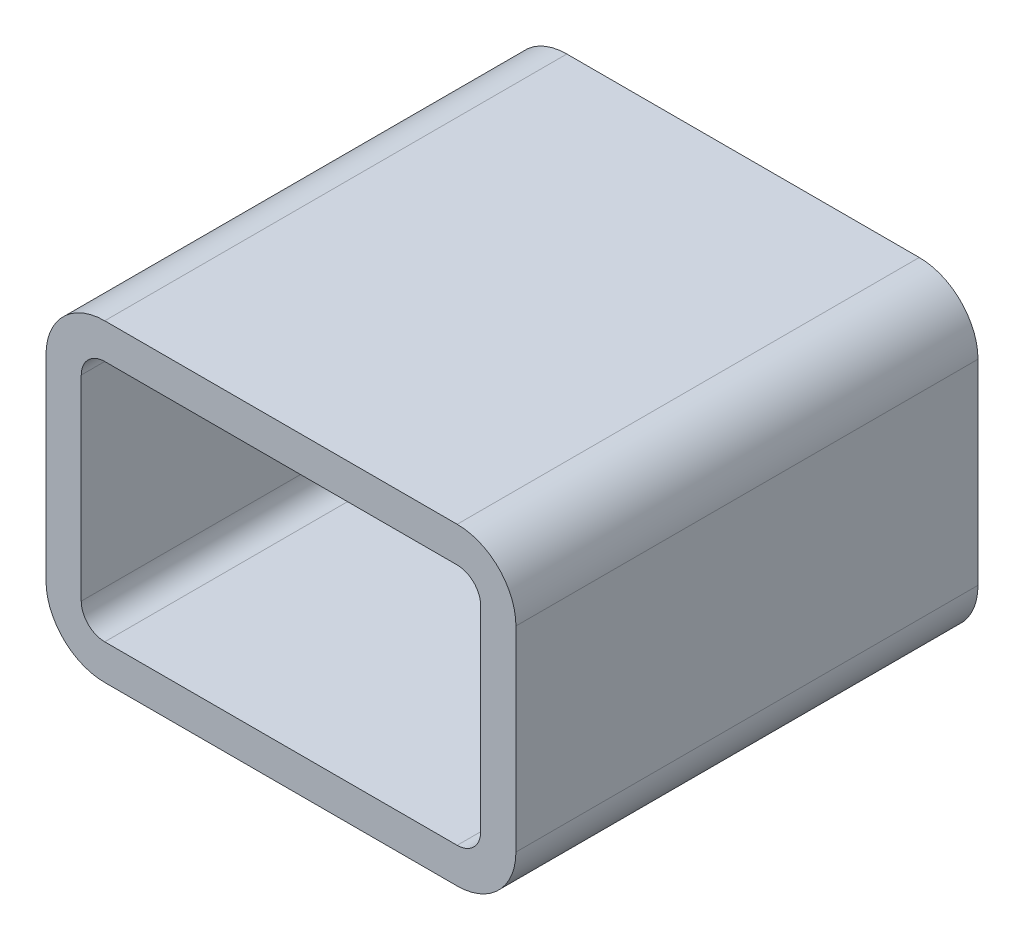
SolidWorks part; units mm, degrees
material "普通碳钢"
ref_plane "前视基准面" through (0, 0, 0) normal (0, 0, 1) x (1, 0, 0)
ref_plane "上视基准面" through (0, 0, 0) normal (0, 1, 0) x (1, 0, 0)
ref_plane "右视基准面" through (0, 0, 0) normal (1, 0, 0) x (0, 0, -1)
sketch "草图1" plane through (0, 0, 0) normal (0, 0, 1) x (1, 0, 0)
  line L0 (-101.745, 0) -> (99.7101, 0) construction
  line L1 (0, 68.9021) -> (0, -49.677) construction
  line L2 (-60, 40) -> (60, 40)
  line L3 (60, 40) -> (60, -40)
  line L4 (60, -40) -> (-60, -40)
  line L5 (-60, -40) -> (-60, 40)
  line L6 (-51, 31) -> (51, 31)
  line L7 (51, 31) -> (51, -31)
  line L8 (51, -31) -> (-51, -31)
  line L9 (-51, -31) -> (-51, 31)
  dimension "D1" = 9
  dimension "D2" = 120
  dimension "D3" = 80
extrude "凸台-拉伸1" add sketch "草图1" along normal blind 118
fillet "圆角1" radius 15 4 edges at (-60, -40, 59) (-60, 40, 59) (60, -40, 59) (60, 40, 59)
fillet "圆角2" radius 6 4 edges at (51, 31, 59) (51, -31, 59) (-51, -31, 59) (-51, 31, 59)
